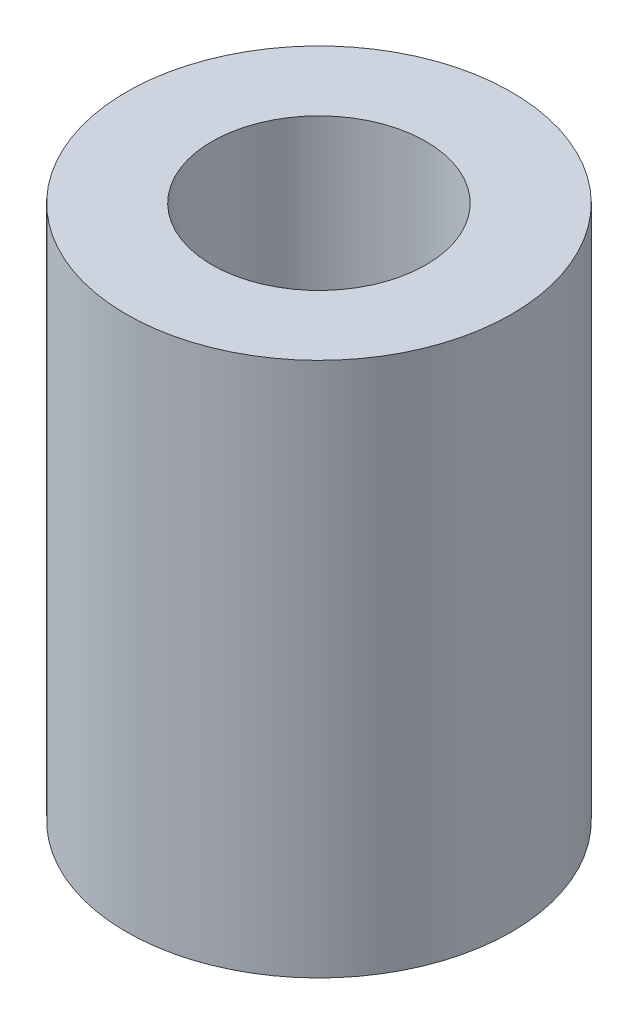
SolidWorks part; units mm, degrees
material "Plain Carbon Steel"
ref_plane "Front Plane" through (0, 0, 0) normal (0, 0, 1) x (1, 0, 0)
ref_plane "Top Plane" through (0, 0, 0) normal (0, 1, 0) x (1, 0, 0)
ref_plane "Right Plane" through (0, 0, 0) normal (1, 0, 0) x (0, 0, -1)
sketch "Sketch1" plane through (0, 0, 0) normal (0, 0, 1) x (1, 0, 0)
  line L0 (0, -309.7318) -> (0, 15176.8578) construction
  line L2 (5, 25) -> (9, 25)
  line L3 (5, 25) -> (5, 0)
  line L4 (5, 0) -> (9, 0)
  line L5 (9, 25) -> (9, 0)
  dimension "D1" = 5
  dimension "D2" = 9
  dimension "D3" = 25
revolve "Revolve1" add sketch "Sketch1" angle 360 about L0
